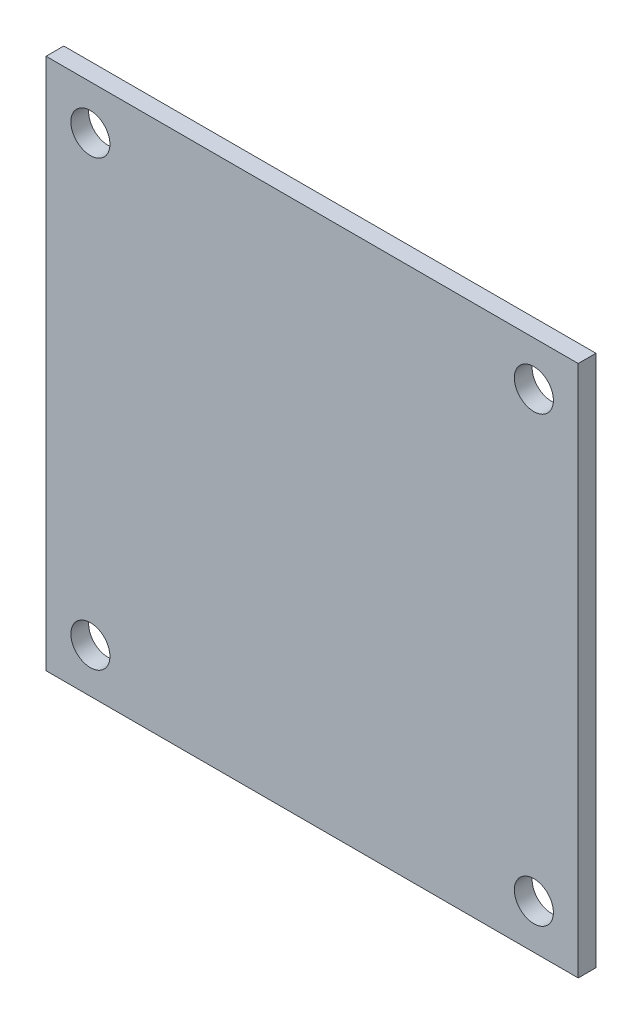
from build123d import *

# Parameters (mm, degrees)
SKETCH1_W           = 300
SKETCH1_H           = 300
SKETCH1_R           = 11
BOSS_EXTRUDE1_DEPTH = 10


with BuildPart() as part:
    # Sketch1 → Boss-Extrude1 (new body)
    with BuildSketch(Plane.XY):
        Rectangle(SKETCH1_W, SKETCH1_H)
        with Locations((-125, 125)):
            Circle(SKETCH1_R, mode=Mode.SUBTRACT)
        with Locations((125, 125)):
            Circle(SKETCH1_R, mode=Mode.SUBTRACT)
        with Locations((125, -125)):
            Circle(SKETCH1_R, mode=Mode.SUBTRACT)
        with Locations((-125, -125)):
            Circle(SKETCH1_R, mode=Mode.SUBTRACT)
    extrude(amount=BOSS_EXTRUDE1_DEPTH)


solid = part.part
